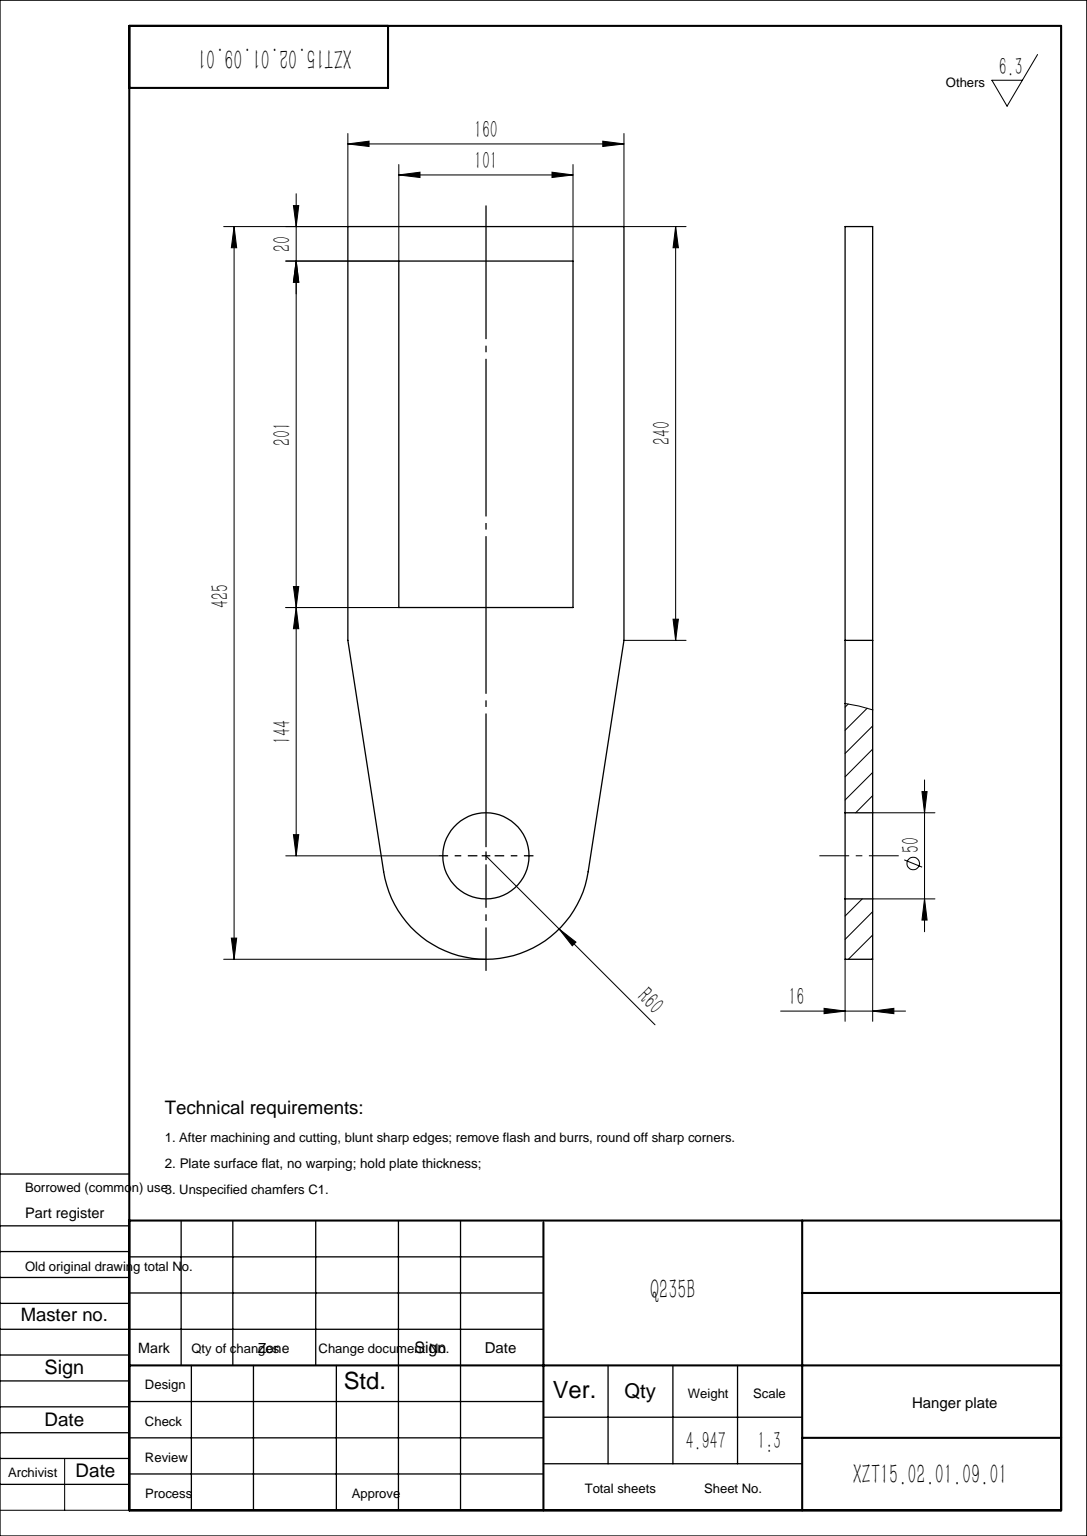
from build123d import *

# Parameters (mm, degrees)
SKETCH1_R           = 25
SKETCH1_W           = 101
SKETCH1_H           = 201
BOSS_EXTRUDE1_DEPTH = 8


with BuildPart() as part:
    # Sketch1 → Boss-Extrude1 (new, symmetric)
    with BuildSketch(Plane.XY):
        with BuildLine():
            Line((80, 365), (-80, 365))
            Line((-80, 365), (-80, 125))
            Line((-80, 125), (-59.298088401, -9.150776577))
            ThreePointArc((-59.298088401, -9.150776577), (-39.057351455, -45.546935103), (0, -60))
            ThreePointArc((0, -60), (39.057351455, -45.546935103), (59.298088401, -9.150776577))
            Line((59.298088401, -9.150776577), (80, 125))
            Line((80, 125), (80, 365))
        make_face()
        Circle(SKETCH1_R, mode=Mode.SUBTRACT)
        with Locations((0, 244.5)):
            Rectangle(SKETCH1_W, SKETCH1_H, mode=Mode.SUBTRACT)
    extrude(amount=BOSS_EXTRUDE1_DEPTH, both=True)


solid = part.part
